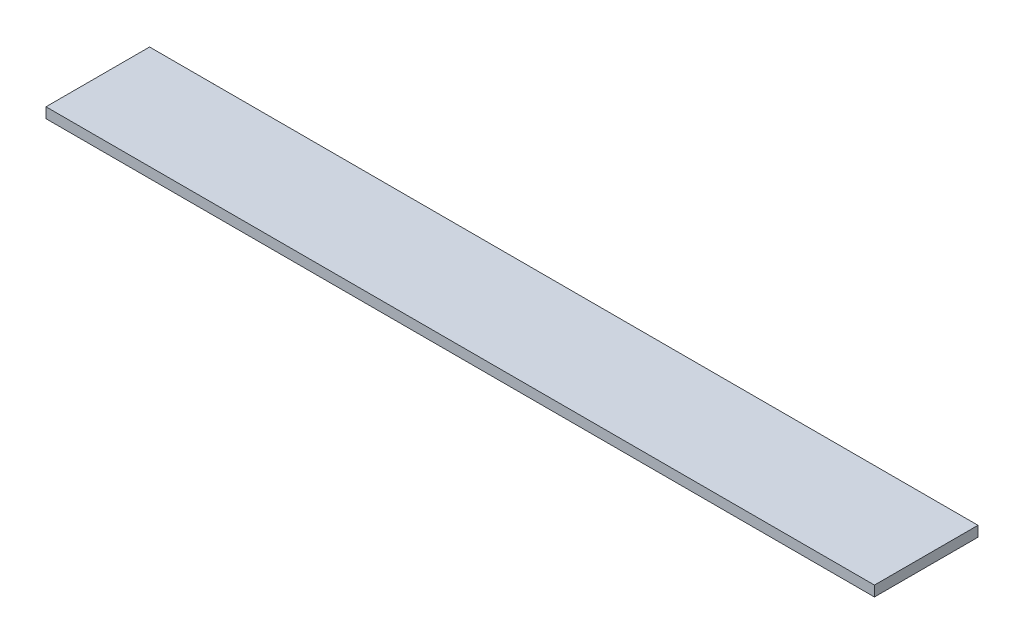
from build123d import *

# Parameters (mm, degrees)
SKETCH1_W           = 400
SKETCH1_H           = 50
BOSS_EXTRUDE1_DEPTH = 5


with BuildPart() as part:
    # Sketch1 → Boss-Extrude1 (new body)
    with BuildSketch(Plane(origin=(0, 0, 0), x_dir=(1, 0, 0), z_dir=(0, 1, 0))):
        Rectangle(SKETCH1_W, SKETCH1_H)
    extrude(amount=BOSS_EXTRUDE1_DEPTH)


solid = part.part
